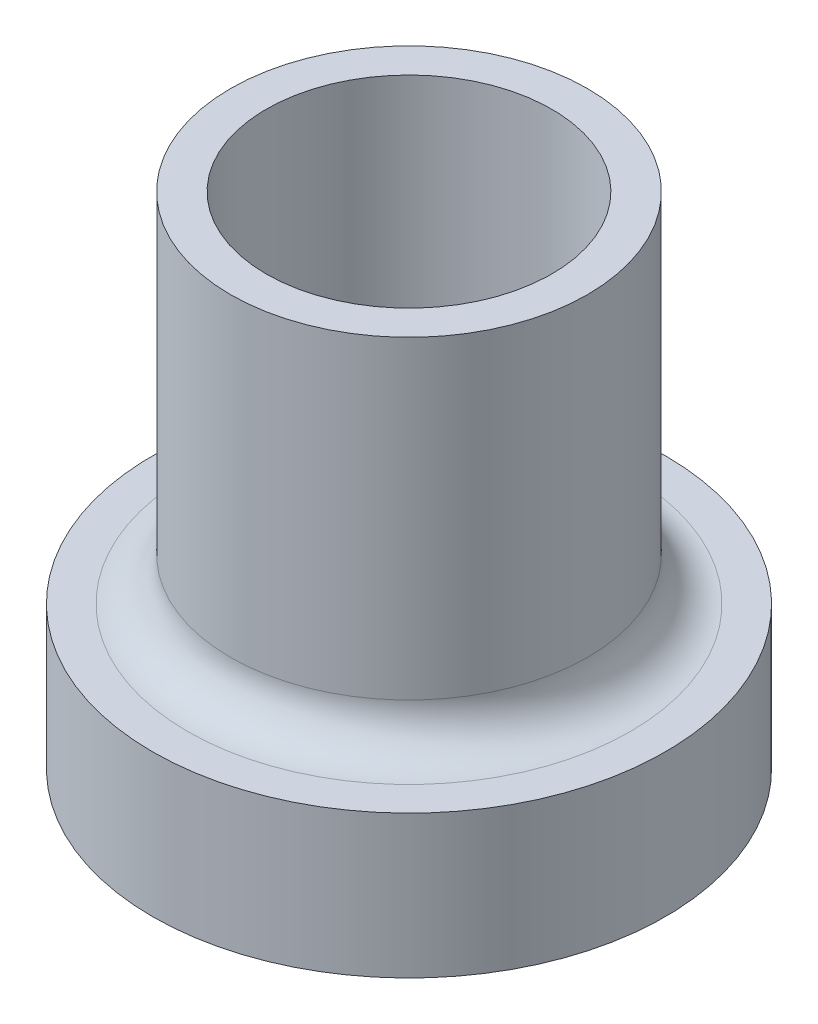
SolidWorks part; units mm, degrees
ref_plane "Front Plane" through (0, 0, 0) normal (0, 0, 1) x (1, 0, 0)
ref_plane "Top Plane" through (0, 0, 0) normal (0, 1, 0) x (1, 0, 0)
ref_plane "Right Plane" through (0, 0, 0) normal (1, 0, 0) x (0, 0, -1)
sketch "Sketch1" plane through (0, 0, 0) normal (0, 0, 1) x (1, 0, 0)
  line L0 (0, 10.8864) -> (0, -11.4318) construction
  line L2 (-10, 28.8368) -> (-12.5, 28.8368)
  line L3 (-10, 28.8368) -> (-10, 1.8368)
  line L5 (-12.5, 28.8368) -> (-12.5, 6.8368)
  line L6 (-15.5, 3.8368) -> (-17.9563, 3.8368)
  line L8 (-15.5, -6.1632) -> (-17.9563, -6.1632)
  line L9 (-17.9563, 3.8368) -> (-17.9563, -6.1632)
  arc A0 (-12.5, 6.8368) -> (-15.5, 3.8368) centre (-15.5, 6.8368) cw
  arc A1 (-10, 1.8368) -> (-15.5, -6.1632) centre (-18.5682, 1.8368) cw
  point P8 (-15.5, -6.1632)
  dimension "D5" = 3
  dimension "D1" = 10
  dimension "D2" = 12.5
  dimension "D3" = 35
  dimension "D4" = 25
  dimension "D6" = 2
revolve "Revolve2" add sketch "Sketch1" angle 360 about L0
